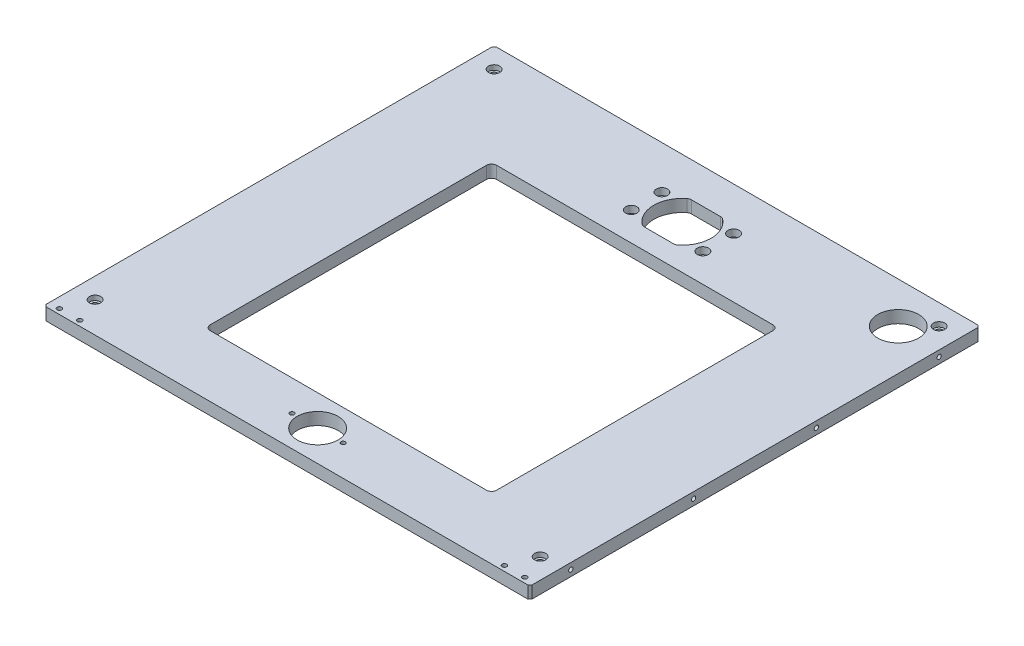
SolidWorks part; units mm, degrees
material "A5052"
ref_plane "Front Plane" through (0, 0, 0) normal (0, 0, 1) x (1, 0, 0)
ref_plane "Top Plane" through (0, 0, 0) normal (0, 1, 0) x (1, 0, 0)
ref_plane "Right Plane" through (0, 0, 0) normal (1, 0, 0) x (0, 0, -1)
sketch "Sketch1" plane through (0, 0, 0) normal (0, 1, 0) x (1, 0, 0)
  line L1 (-237.5, 220) -> (237.5, 220)
  line L2 (-237.5, 220) -> (-237.5, -220)
  line L3 (-237.5, -220) -> (237.5, -220)
  line L4 (237.5, 220) -> (237.5, -220)
  line L5 (-237.5, 220) -> (237.5, -220) construction
  line L6 (-237.5, -220) -> (237.5, 220) construction
  point P0 (0, 0)
  dimension "D1" = 475
  dimension "D2" = 440
extrude "Boss-Extrude1" add sketch "Sketch1" along normal blind 12
sketch "Sketch3" plane through (0, 12, 0) normal (0, 1, 0) x (1, 0, 0)
  line L0 (0, 0) -> (0, -190) construction
  line L1 (-237.5, -220) -> (237.5, -220) construction
  circle A0 centre (0, -190) radius 20
  dimension "D1" = 30
  dimension "D2" = 40
extrude "Cut-Extrude2" cut sketch "Sketch3" against normal through all
hole_wizard "Hex socket button head screw hole 1" positions "Sketch32" profile "Sketch31" counterbore size "M6" standard "GB" end condition through all
sketch "Sketch32" plane through (0, 12, 0) normal (0, 1, 0) x (1, 0, 0)
  line L16 (217.5, -190) -> (217.5, 200) construction
  line L17 (217.5, 200) -> (-217.5, 200) construction
  line L18 (-217.5, 200) -> (-217.5, -190) construction
  line L21 (-237.5, 220) -> (-237.5, -220) construction
  line L22 (217.5, -190) -> (-217.5, -190) construction
  line L24 (-237.5, -220) -> (237.5, -220) construction
  line L25 (237.5, -220) -> (237.5, 220) construction
  line L26 (237.5, 220) -> (-237.5, 220) construction
  point P0 (217.5, 200)
  point P46 (217.5, -190)
  point P49 (-217.5, -190)
  point P52 (-217.5, 200)
  dimension "D2" = 20
  dimension "D3" = 30
  dimension "D1" = 20
  dimension "D4" = 20
sketch "Sketch31" plane through (217.5, 12, -200) normal (1, 0, 0) x (0, 0, 1)
  line L0 (0, 0) -> (0, 12)
  line L1 (0, 12) -> (3.3, 12)
  line L3 (3.3, 12) -> (3.3, 4.7)
  line L4 (3.3, 4.7) -> (5.5, 4.7)
  line L5 (5.5, 4.7) -> (5.5, 0)
  line L7 (5.5, 0) -> (0, 0)
  line L11 (0, -6.35) -> (0, 107.95) construction
  dimension "通孔孔直径" = 6.6
  dimension "通孔孔深度" = 12
  dimension "柱形沉头孔直径" = 11
  dimension "柱形沉头孔深度" = 4.7
chamfer "Chamfer1" distance 2 angle 45 4 edges at (-237.5, 6, 220) (-237.5, 6, -220) (237.5, 6, -220) (237.5, 6, 220)
sketch "Sketch33" plane through (0, 12, 0) normal (0, 1, 0) x (1, 0, 0)
  line L0 (19.2329, 141) -> (-12.0721, 141) construction
  line L1 (-12.0721, 185) -> (19.2329, 185) construction
  line L2 (19.2329, 141) -> (-12.0721, 141) construction
  line L3 (-12.0721, 185) -> (19.2329, 185) construction
  line L4 (-12.3883, 186) -> (19.5491, 186)
  line L5 (19.5491, 140) -> (-12.3883, 140)
  arc A0 (19.2329, 141) -> (19.2329, 185) centre (3.5804, 163) ccw construction
  arc A1 (-12.0721, 185) -> (-12.0721, 141) centre (3.5804, 163) ccw construction
  arc A2 (19.2329, 141) -> (19.2329, 185) centre (3.5804, 163) ccw construction
  arc A3 (-12.0721, 185) -> (-12.0721, 141) centre (3.5804, 163) ccw construction
  arc A4 (19.5491, 140) -> (19.5491, 186) centre (3.5804, 163) ccw
  arc A5 (-12.3883, 186) -> (-12.3883, 140) centre (3.5804, 163) ccw
  dimension "D1" = 1
extrude "Cut-Extrude4" cut sketch "Sketch33" against normal up to next
hole_wizard "Hex socket cap screw hole type 1" positions "Sketch34" profile "Sketch35" counterbore size "M6" standard "GB" end condition up to next
sketch "Sketch34" plane through (0, 12, 0) normal (0, 1, 0) x (1, 0, 0)
  line L1 (3.5804, 140) -> (3.5804, 184.594) construction
  line L2 (-12.3883, 140) -> (19.5491, 140) construction
  point P0 (38.5804, 148)
  point P2 (38.5804, 178)
  point P5 (-31.4196, 148)
  point P7 (-31.4196, 178)
  dimension "D1" = 30
  dimension "D2" = 70
  dimension "D3" = 8
sketch "Sketch35" plane through (38.5804, 12, -148) normal (1, 0, 0) x (0, 0, 1)
  line L0 (0, 0) -> (0, 12)
  line L1 (0, 12) -> (3.3, 12)
  line L3 (3.3, 12) -> (3.3, 6.8)
  line L4 (3.3, 6.8) -> (5.5, 6.8)
  line L5 (5.5, 6.8) -> (5.5, 0)
  line L7 (5.5, 0) -> (0, 0)
  line L11 (0, -6.35) -> (0, 107.95) construction
  dimension "通孔孔直径" = 6.6
  dimension "通孔孔深度" = 12
  dimension "柱形沉头孔直径" = 11
  dimension "柱形沉头孔深度" = 6.8
fillet "Fillet1" radius 5 4 edges at (19.5491, 6, -140) (-12.3883, 6, -140) (-12.3883, 6, -186) (19.5491, 6, -186)
hole_wizard "M5 Tapped Hole1" positions "Sketch36" profile "Sketch37" tap size "M5" standard "GB" end condition up to next
sketch "Sketch36" plane through (0, 12, 0) normal (0, 1, 0) x (1, 0, 0)
  point P0 (-25, -190)
  point P3 (25, -190)
sketch "Sketch37" plane through (-25, 12, 190) normal (1, 0, 0) x (0, 0, 1)
  line L0 (0, 0) -> (0, 12)
  line L1 (0, 12) -> (2.1, 12)
  line L2 (2.1, 12) -> (2.1, 0)
  line L5 (2.1, 0) -> (0, 0)
  line L11 (0, -6.35) -> (0, 107.95) construction
  dimension "通孔螺纹孔钻头直径" = 4.2
  dimension "通孔螺纹孔钻头深度" = 12
cosmetic thread "Hole thread 1" parameters "D2"=5
cosmetic thread "Hole thread 2" parameters "D2"=5
hole_wizard "M5 Tapped Hole2" positions "Sketch38" profile "Sketch39" tap size "M5" standard "GB"
sketch "Sketch38" plane through (-237.5, 0, 0) normal (-1, 0, 0) x (0, 0, 1)
  line L1 (218, 0) -> (218, 12) construction
  line L2 (0, 0) -> (0, 12) construction
  line L3 (-218, 0) -> (218, 0) construction
  line L4 (-218, 12) -> (218, 12) construction
  point P0 (-180, 6)
  point P2 (-60, 6)
  point P4 (60, 6)
  point P6 (180, 6)
  point P15 (218, 6)
  dimension "D1" = 120
  dimension "D2" = 120
sketch "Sketch39" plane through (-237.5, 6, -180) normal (0, 1, 0) x (0, 0, 1)
  line L0 (0, 0) -> (0, 15.2618)
  line L1 (0, 15.2618) -> (2.1, 14)
  line L2 (2.1, 14) -> (2.1, 0)
  line L5 (2.1, 0) -> (0, 0)
  line L10 (0, 15.2618) -> (-2.1, 14) construction
  line L11 (0, -6.35) -> (0, 107.95) construction
  dimension "螺纹孔钻头直径" = 4.2
  dimension "螺纹孔钻头深度" = 14
  dimension "导头角度" = 118
cosmetic thread "Hole thread 3" parameters "D1"=10, "D2"=5
cosmetic thread "Hole thread 4" parameters "D1"=10, "D2"=5
cosmetic thread "Hole thread 5" parameters "D1"=10, "D2"=5
cosmetic thread "Hole thread 6" parameters "D1"=10, "D2"=5
mirror "Mirror1" about plane through (0, 0, 0) normal (1, 0, 0) of "M5 Tapped Hole2"
hole_wizard "M5 Tapped Hole3" positions "Sketch40" profile "Sketch41" tap size "M5" standard "GB"
sketch "Sketch40" plane through (0, 0, -220) normal (0, 0, -1) x (-1, 0, 0)
  line L0 (-235.5, 12) -> (-235.5, 0) construction
  line L1 (0, 0) -> (0, 14.0111) construction
  line L2 (-235.5, 0) -> (235.5, 0) construction
  point P0 (-195, 6)
  point P2 (-65, 6)
  point P4 (65, 6)
  point P6 (195, 6)
  point P12 (-235.5, 6)
  dimension "D1" = 130
  dimension "D2" = 130
sketch "Sketch41" plane through (195, 6, -220) normal (1, 0, 0) x (0, 1, 0)
  line L0 (0, 0) -> (0, 15.2618)
  line L1 (0, 15.2618) -> (2.1, 14)
  line L2 (2.1, 14) -> (2.1, 0)
  line L5 (2.1, 0) -> (0, 0)
  line L10 (0, 15.2618) -> (-2.1, 14) construction
  line L11 (0, -6.35) -> (0, 107.95) construction
  dimension "螺纹孔钻头直径" = 4.2
  dimension "螺纹孔钻头深度" = 14
  dimension "导头角度" = 118
cosmetic thread "Hole thread 7" parameters "D1"=10, "D2"=5
cosmetic thread "Hole thread 8" parameters "D1"=10, "D2"=5
cosmetic thread "Hole thread 9" parameters "D1"=10, "D2"=5
cosmetic thread "Hole thread 10" parameters "D1"=10, "D2"=5
hole_wizard "M4 Clearance Hole1" positions "Sketch44" profile "Sketch45" hole size "M4" standard "GB" end condition up to next
sketch "Sketch44" plane through (0, 12, 0) normal (0, 1, 0) x (1, 0, 0)
  point P0 (-227.5, -215)
  point P3 (-207.5, -215)
  point P6 (207.5, -215)
  point P9 (227.5, -215)
sketch "Sketch45" plane through (-227.5, 12, 215) normal (1, 0, 0) x (0, 0, 1)
  line L0 (0, 0) -> (0, 12)
  line L1 (0, 12) -> (2.25, 12)
  line L2 (2.25, 12) -> (2.25, 0)
  line L5 (2.25, 0) -> (0, 0)
  line L11 (0, -6.35) -> (0, 107.95) construction
  dimension "通孔孔直径" = 4.5
  dimension "通孔孔深度" = 12
sketch "Sketch46" plane through (0, 12, 0) normal (0, 1, 0) x (1, 0, 0)
  line L0 (235.5, 220) -> (-235.5, 220) construction
  line L1 (140, -160) -> (-140, -160)
  line L2 (140, -160) -> (140, 120)
  line L3 (140, 120) -> (-140, 120)
  line L4 (-140, -160) -> (-140, 120)
  line L5 (140, -160) -> (-140, 120) construction
  line L6 (140, 120) -> (-140, -160) construction
  line L7 (0, 220) -> (0, 30.2105) construction
  point P0 (0, 0)
  dimension "D1" = 280
  dimension "D2" = 280
  dimension "D3" = 100
extrude "Cut-Extrude5" cut sketch "Sketch46" against normal through all
fillet "Fillet2" radius 5 4 edges at (140, 6, -120) (-140, 6, -120) (-140, 6, 160) (140, 6, 160)
sketch "Sketch47" plane through (0, 12, 0) normal (0, 1, 0) x (1, 0, 0)
  line L0 (235.5, 220) -> (-235.5, 220) construction
  line L1 (237.5, -218) -> (237.5, 218) construction
  circle A0 centre (197.5, 180) radius 20
  dimension "D1" = 40
  dimension "D2" = 40
  dimension "D3" = 40
extrude "Cut-Extrude6" cut sketch "Sketch47" against normal through all
